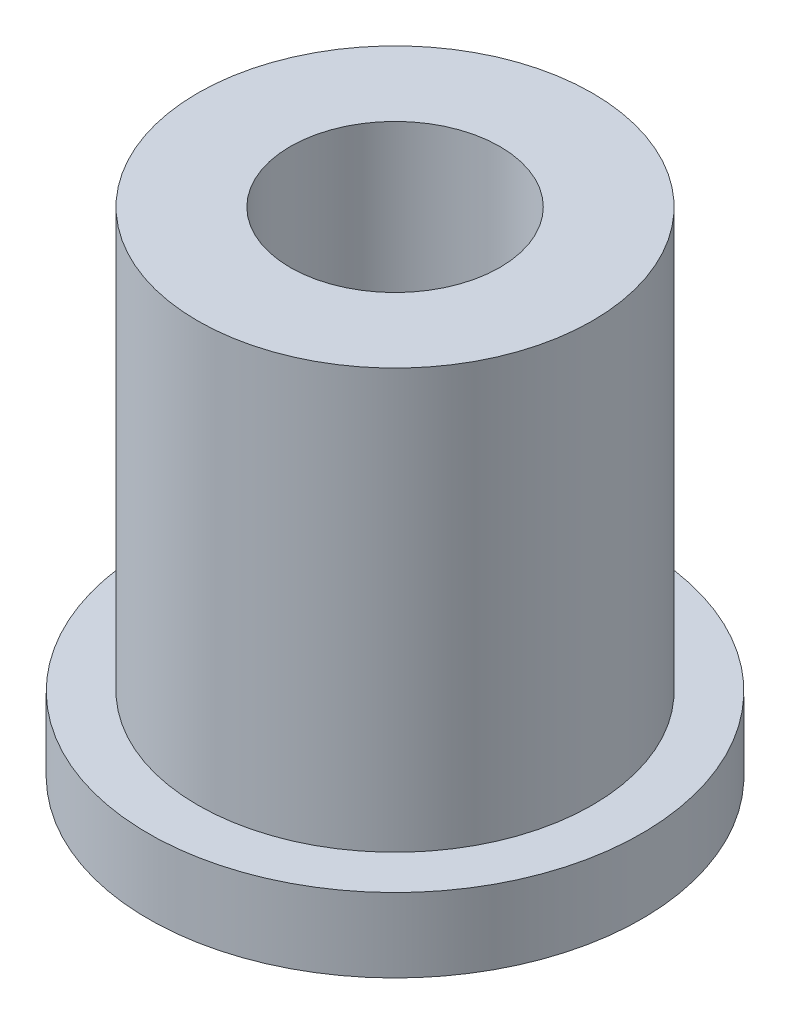
from build123d import *

# Parameters (mm, degrees)
SKETCH1_R              = 8
BOSS_EXTRUDE1_DEPTH    = 20
M10_TAPPED_HOLE1_D     = 8.5
M10_TAPPED_HOLE1_DEPTH = 24.5
M10_TAPPED_HOLE1_TIP   = 2.553657631
SKETCH4_R              = 10
SKETCH4_R_2            = 8
BOSS_EXTRUDE3_DEPTH    = 3


with BuildPart() as part:
    # Sketch1 → Boss-Extrude1 (new body)
    with BuildSketch(Plane(origin=(0, 0, 0), x_dir=(1, 0, 0), z_dir=(0, 1, 0))):
        with Locations(Location((0, 0, 0), (0, 0, 270))):
            Circle(SKETCH1_R)
    extrude(amount=BOSS_EXTRUDE1_DEPTH)

    # M10 Tapped Hole1
    with Locations(Plane(origin=(0, 20, 0), x_dir=(1, 0, 0), z_dir=(0, 1, 0))):
        with Locations((0, 0)):
            Hole(M10_TAPPED_HOLE1_D / 2, depth=M10_TAPPED_HOLE1_DEPTH)
            with Locations((0, 0, -(M10_TAPPED_HOLE1_DEPTH + M10_TAPPED_HOLE1_TIP / 2))):  # 118° drill point
                Cone(0, M10_TAPPED_HOLE1_D / 2, M10_TAPPED_HOLE1_TIP, mode=Mode.SUBTRACT)

    # Sketch4 → Boss-Extrude3 (add)
    with BuildSketch(Plane.XZ):
        with Locations(Location((0, 0, 0), (0, 0, 270))):
            Circle(SKETCH4_R)
        with Locations(Location((0, 0, 0), (0, 0, 270))):
            Circle(SKETCH4_R_2, mode=Mode.SUBTRACT)
    extrude(amount=-BOSS_EXTRUDE3_DEPTH)


solid = part.part
